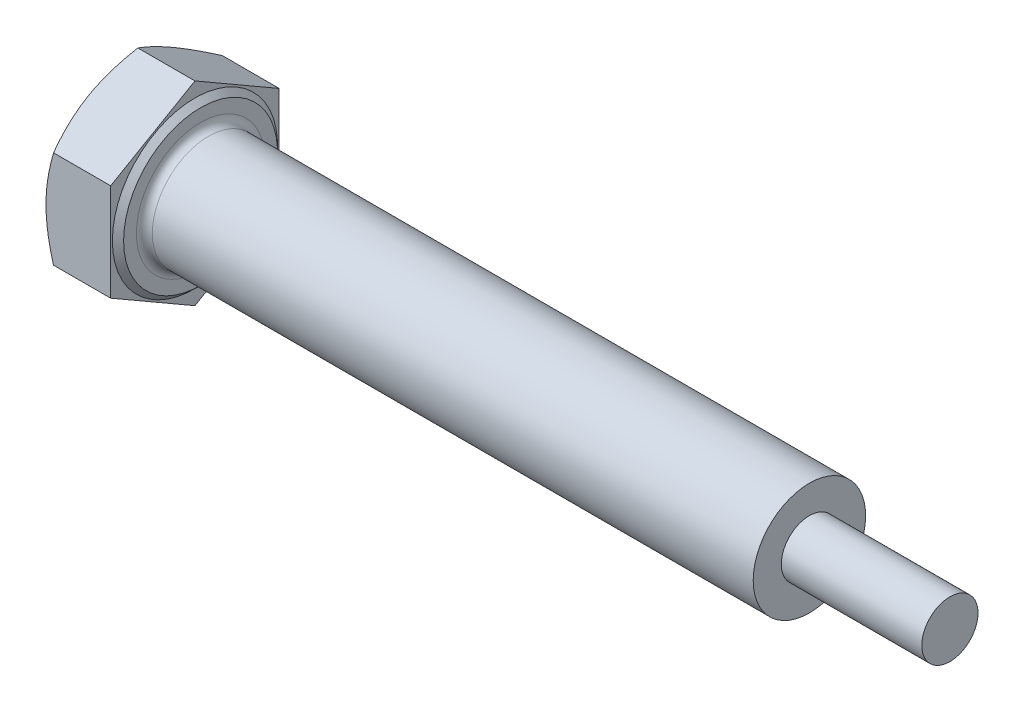
from build123d import *

# Parameters (mm, degrees)
BOSS_EXTRUDE1_DEPTH = 7.5
SKETCH4_R           = 20.03
SKETCH4_R_2         = 9
CUT_EXTRUDE1_DEPTH  = 0.9375
CUT_EXTRUDE1_DRAFT  = -60
CHAMFER2_SIZE       = 0.666666667
SKETCH9_R           = 8.815
SKETCH9_R_2         = 3
CUT_EXTRUDE2_DEPTH  = 15


with BuildPart() as part:
    # Sketch3 → Boss-Extrude1 (new body)
    with BuildSketch(Plane(origin=(0, 0, 0), x_dir=(0, 0, -1), z_dir=(1, 0, 0))):
        Polygon((9, 5.196152423), (0, 10.392304845), (-9, 5.196152423), (-9, -5.196152423), (0, -10.392304845), (9, -5.196152423), align=None)
    extrude(amount=BOSS_EXTRUDE1_DEPTH)


with BuildPart() as cut_extrude1_tool:
    # Sketch4 → Cut-Extrude1 (with draft: the straight prism first)
    with BuildSketch(Plane.ZY):
        Circle(SKETCH4_R)
        Circle(SKETCH4_R_2, mode=Mode.SUBTRACT)
    extrude(amount=-CUT_EXTRUDE1_DEPTH)
    # Cut-Extrude1: the draft: its side faces are tilted about the plane it starts from
    cut_extrude1_sides = [cut_extrude1_tool.faces().sort_by_distance(p)[0] for p in [
        (0.46875, 0, -20.03),
        (0.46875, 0, -9),
    ]]
    draft(cut_extrude1_sides, Plane.ZY, CUT_EXTRUDE1_DRAFT)


with BuildPart() as part_1:
    add(part.part)

    # Cut-Extrude1: cut by cut_extrude1_tool
    add(cut_extrude1_tool.part, mode=Mode.SUBTRACT)

    # Sketch5 → Revolve1 (revolve)
    with BuildSketch(Plane.XY, mode=Mode.PRIVATE) as revolve1_sk:
        with BuildLine():
            Line((8.35, 6), (87.5, 6))
            Line((87.5, 6), (87.5, 0))
            Line((87.5, 0), (7.5, 0))
            Line((7.5, 0), (7.5, 6.85))
            ThreePointArc((7.5, 6.85), (7.748959236, 6.248959236), (8.35, 6))
        make_face()
    revolve(revolve1_sk.sketch.rotate(Axis((7.5, 0, 0), (1, 0, 0)), 90), axis=Axis((7.5, 0, 0), (1, 0, 0)))

    # Chamfer2
    chamfer2_edges = [part_1.edges().sort_by_distance(p)[0] for p in [
        (87.5, 0, -6),
    ]]
    chamfer(chamfer2_edges, length=CHAMFER2_SIZE)

    # Sketch7 → Cut-Revolve1 (revolve, cut)
    with BuildSketch(Plane.XY, mode=Mode.PRIVATE) as cut_revolve1_sk:
        Polygon((7.5, 8.215), (6.9, 8.815), (6.9, 20.03), (7.5, 20.03), align=None)
    revolve(cut_revolve1_sk.sketch.rotate(Axis((0, 0, 0), (1, 0, 0)), 90), axis=Axis((0, 0, 0), (1, 0, 0)), mode=Mode.SUBTRACT)

    # Sketch9 → Cut-Extrude2 (cut)
    with BuildSketch(Plane(origin=(87.5, 0, 0), x_dir=(0, 0, -1), z_dir=(1, 0, 0))):
        Circle(SKETCH9_R)
        Circle(SKETCH9_R_2, mode=Mode.SUBTRACT)
    extrude(amount=-CUT_EXTRUDE2_DEPTH, mode=Mode.SUBTRACT)


solid = part_1.part
